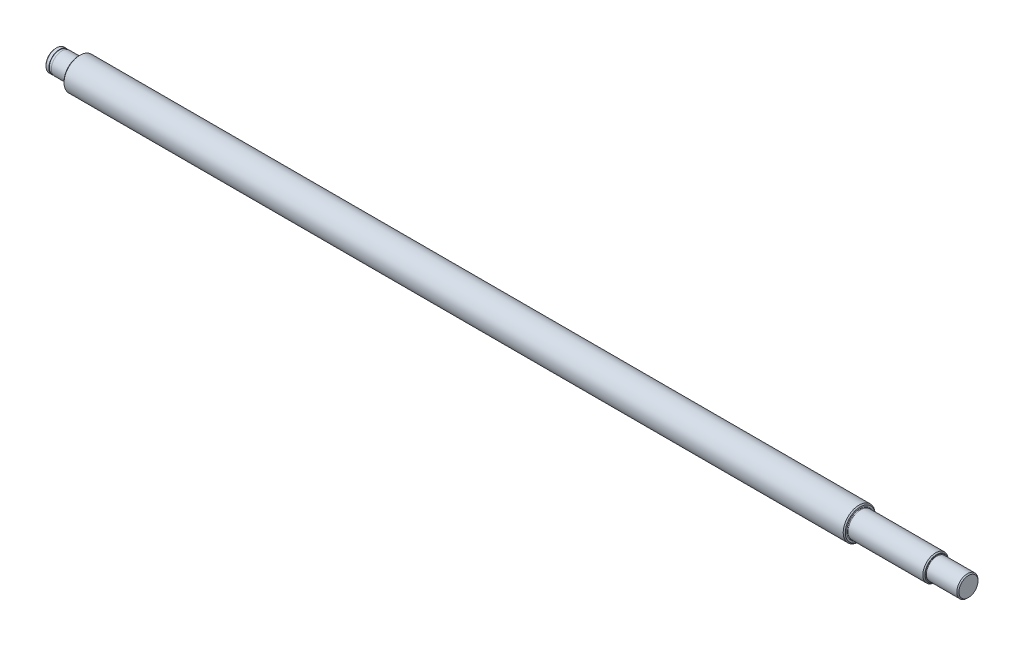
from build123d import *


with BuildPart() as part:
    # Sketch1 → Revolve1 (revolve)
    with BuildSketch(Plane.XY, mode=Mode.PRIVATE) as revolve1_sk:
        with BuildLine():
            Line((1.85, 5), (1.85, 4.8))
            Line((1.85, 4.8), (3, 4.8))
            Line((3, 4.8), (3, 5))
            Line((3, 5), (10.7, 5))
            ThreePointArc((10.7, 5), (10.912132034, 5.087867966), (11, 5.3))
            Line((11, 5.3), (11, 7))
            Line((11, 7), (11.5, 7.5))
            Line((11.5, 7.5), (378.5, 7.5))
            Line((378.5, 7.5), (379, 7))
            Line((379, 7), (379, 6.3))
            ThreePointArc((379, 6.3), (379.087867966, 6.087867966), (379.3, 6))
            Line((379.3, 6), (414.5, 6))
            Line((414.5, 6), (415, 5.5))
            Line((415, 5.5), (415, 5.2))
            ThreePointArc((415, 5.2), (415.058578644, 5.058578644), (415.2, 5))
            Line((415.2, 5), (429.5, 5))
            Line((429.5, 5), (430, 4.5))
            Line((430, 4.5), (430, 0))
            Line((430, 0), (0, 0))
            Line((0, 0), (0, 4.5))
            Line((0, 4.5), (0.5, 5))
            Line((0.5, 5), (1.85, 5))
        make_face()
    revolve(revolve1_sk.sketch.rotate(Axis((-7.5, 0, 0), (1, 0, 0)), 90), axis=Axis((-7.5, 0, 0), (1, 0, 0)))


solid = part.part
